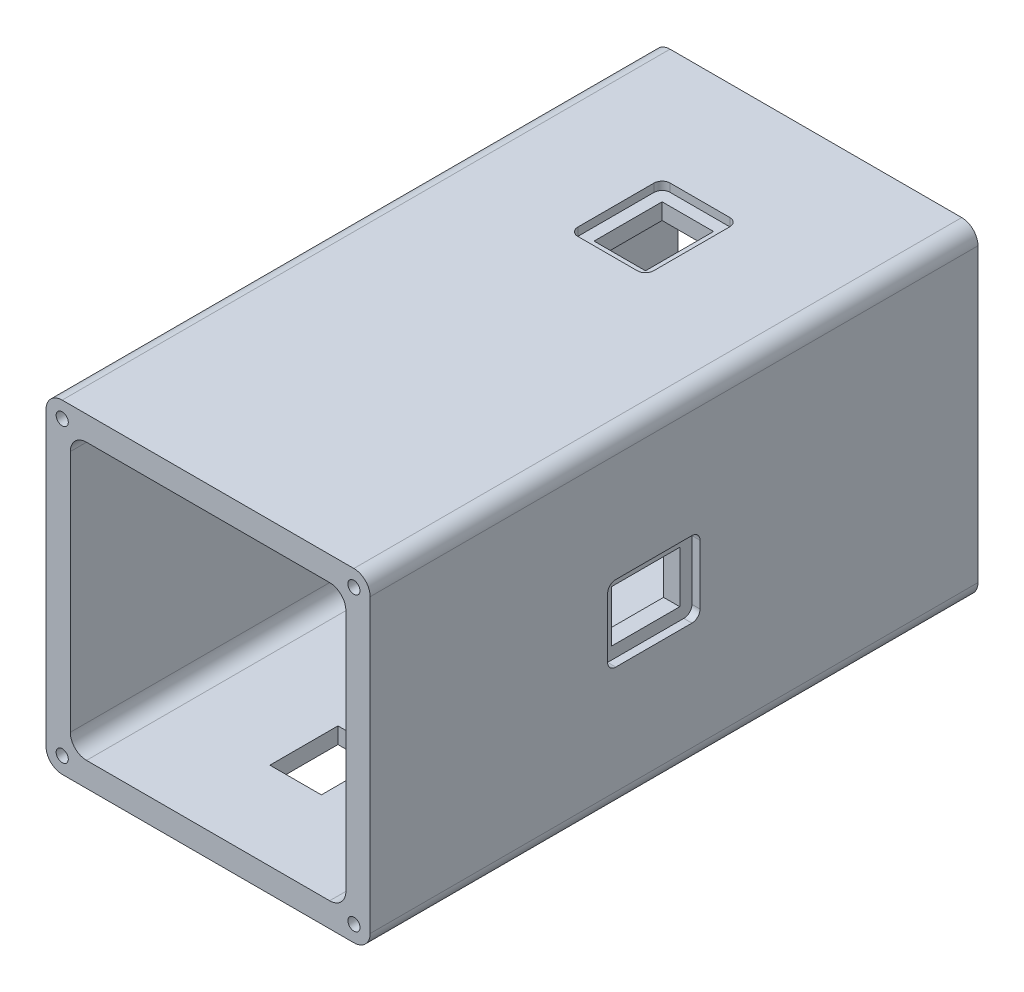
SolidWorks part; units mm, degrees
ref_plane "Front Plane" through (0, 0, 0) normal (0, 0, 1) x (1, 0, 0)
ref_plane "Top Plane" through (0, 0, 0) normal (0, 1, 0) x (1, 0, 0)
ref_plane "Right Plane" through (0, 0, 0) normal (1, 0, 0) x (0, 0, -1)
sketch "Sketch1" plane through (0, 0, 0) normal (0, 0, 1) x (1, 0, 0)
  line L104 (10.5727, 43.58) -> (10.5727, -28.42)
  line L117 (14.5727, -32.42) -> (86.5726, -32.42)
  line L130 (90.5727, -28.4199) -> (90.5727, 43.5589)
  line L143 (86.5517, 47.58) -> (14.5726, 47.58)
  line L212 (16.5727, 37.58) -> (16.5727, -22.42)
  line L213 (20.5727, -26.42) -> (80.5726, -26.42)
  line L214 (84.5726, -22.42) -> (84.5726, 37.58)
  line L215 (80.5726, 41.58) -> (20.5727, 41.58)
  arc A0 (90.5727, 43.5589) -> (86.5517, 47.58) centre (86.5517, 43.5589) ccw
  arc A1 (10.5727, -28.42) -> (14.5727, -32.42) centre (14.5727, -28.42) ccw
  arc A2 (10.5727, 43.58) -> (14.5726, 47.58) centre (14.5726, 43.58) cw
  arc A3 (86.5726, -32.42) -> (90.5727, -28.4199) centre (86.5726, -28.4199) ccw
  arc A4 (80.5726, -26.42) -> (84.5726, -22.42) centre (80.5726, -22.42) ccw
  arc A5 (84.5726, 37.58) -> (80.5726, 41.58) centre (80.5726, 37.58) ccw
  arc A6 (16.5727, 37.58) -> (20.5727, 41.58) centre (20.5727, 37.58) cw
  arc A7 (16.5727, -22.42) -> (20.5727, -26.42) centre (20.5727, -22.42) ccw
  dimension "D1" = 4
extrude "Boss-Extrude1" add sketch "Sketch1" along normal up to surface (150 mm away)
sketch "Sketch2" plane through (0, 0, 150) normal (0, 0, 1) x (1, 0, 0)
  circle A0 centre (14.5727, -28.42) radius 1.5
  circle A1 centre (14.5726, 43.58) radius 1.5
  circle A2 centre (86.5517, 43.5589) radius 1.5003
  circle A3 centre (86.5726, -28.4199) radius 1.5
extrude "Cut-Extrude1" cut sketch "Sketch2" against normal blind 5
ref_plane "Plane1" through (0, 0, 75) normal (0, 0, -1) x (-1, 0, 0)
mirror "Mirror1" about plane through (0, 0, 75) normal (0, 0, -1) of "Cut-Extrude1"
ref_plane "Plane3" through (50.5727, 0, 0) normal (-1, 0, 0) x (0, 0, 1)
sketch "Sketch7" plane through (0, 47.58, 0) normal (0, 1, 0) x (1, 0, 0)
  line L0 (50.5622, -31.6) -> (50.5622, 0) construction
  line L1 (56.9122, -48.4) -> (44.2122, -48.4)
  line L2 (56.9122, -48.4) -> (56.9122, -31.6)
  line L3 (56.9122, -31.6) -> (44.2122, -31.6)
  line L4 (44.2122, -48.4) -> (44.2122, -31.6)
  line L5 (86.5517, 0) -> (14.5726, 0) construction
  line L6 (56.9122, -40) -> (44.2122, -40) construction
  dimension "D1" = 16.8
  dimension "D2" = 12.7
  dimension "D3" = 40
extrude "Cut-Extrude2" cut sketch "Sketch7" against normal blind 13
sketch "Sketch8" plane through (90.5727, 0, 0) normal (1, 0, 0) x (0, 0, -1)
  line L0 (-71.6, 7.5695) -> (-150, 7.5695) construction
  line L1 (-71.6, 13.9195) -> (-71.6, 1.2195)
  line L2 (-71.6, 13.9195) -> (-88.4, 13.9195)
  line L3 (-88.4, 13.9195) -> (-88.4, 1.2195)
  line L4 (-71.6, 1.2195) -> (-88.4, 1.2195)
  line L5 (-80, 13.9195) -> (-80, 1.2195) construction
  line L6 (-150, -28.4199) -> (-150, 43.5589) construction
  line L7 (0, -28.4199) -> (0, 43.5589) construction
  dimension "D1" = 16.8
  dimension "D2" = 12.7
  dimension "D3" = 78.4
  dimension "D4" = 80
extrude "Cut-Extrude3" cut sketch "Sketch8" against normal blind 13
sketch "Sketch9" plane through (0, -32.42, 0) normal (0, -1, 0) x (1, 0, 0)
  line L0 (50.5726, 128.4) -> (50.5726, 150) construction
  line L1 (56.9226, 111.6) -> (44.2226, 111.6)
  line L2 (56.9226, 111.6) -> (56.9226, 128.4)
  line L3 (56.9226, 128.4) -> (44.2226, 128.4)
  line L4 (44.2226, 111.6) -> (44.2226, 128.4)
  line L5 (56.9226, 120) -> (44.2226, 120) construction
  line L6 (14.5727, 150) -> (86.5726, 150) construction
  line L7 (14.5727, 0) -> (86.5726, 0) construction
  dimension "D1" = 16.8
  dimension "D2" = 12.7
  dimension "D3" = 120
extrude "Cut-Extrude4" cut sketch "Sketch9" against normal blind 13
sketch "Sketch10" plane through (0, 47.58, 0) normal (0, 1, 0) x (1, 0, 0)
  line L9 (59.9122, -28.6) -> (41.2122, -28.6)
  line L10 (41.2122, -28.6) -> (41.2122, -51.4)
  line L11 (41.2122, -51.4) -> (59.9122, -51.4)
  line L12 (59.9122, -51.4) -> (59.9122, -28.6)
  line L13 (59.9122, -28.6) -> (41.2122, -28.6)
  line L14 (41.2122, -28.6) -> (41.2122, -51.4)
  line L15 (41.2122, -51.4) -> (59.9122, -51.4)
  line L16 (59.9122, -51.4) -> (59.9122, -28.6)
  dimension "D1" = 3
extrude "Cut-Extrude5" cut sketch "Sketch10" against normal blind 2
fillet "Fillet1" radius 2 4 edges at (41.2122, 46.58, 51.4) (41.2122, 46.58, 28.6) (59.9122, 46.58, 28.6) (59.9122, 46.58, 51.4)
sketch "Sketch12" plane through (90.5727, 0, 0) normal (1, 0, 0) x (0, 0, -1)
  line L8 (-91.4, 16.9195) -> (-91.4, -1.7805)
  line L9 (-91.4, -1.7805) -> (-68.6, -1.7805)
  line L10 (-68.6, 16.9195) -> (-91.4, 16.9195)
  line L11 (-68.6, -1.7805) -> (-68.6, 16.9195)
  line L12 (-91.4, 16.9195) -> (-91.4, -1.7805)
  line L13 (-91.4, -1.7805) -> (-68.6, -1.7805)
  line L14 (-68.6, 16.9195) -> (-91.4, 16.9195)
  line L15 (-68.6, -1.7805) -> (-68.6, 16.9195)
  dimension "D1" = 3
extrude "Cut-Extrude6" cut sketch "Sketch12" against normal blind 2
fillet "Fillet2" radius 2 4 edges at (89.5727, 16.9195, 68.6) (89.5727, -1.7805, 68.6) (89.5727, 16.9195, 91.4) (89.5727, -1.7805, 91.4)
sketch "Sketch13" plane through (0, -32.42, 0) normal (0, -1, 0) x (1, 0, 0)
  line L8 (41.2226, 108.6) -> (59.9226, 108.6)
  line L9 (41.2226, 131.4) -> (41.2226, 108.6)
  line L10 (59.9226, 108.6) -> (59.9226, 131.4)
  line L11 (59.9226, 131.4) -> (41.2226, 131.4)
  line L12 (41.2226, 108.6) -> (59.9226, 108.6)
  line L13 (41.2226, 131.4) -> (41.2226, 108.6)
  line L14 (59.9226, 108.6) -> (59.9226, 131.4)
  line L15 (59.9226, 131.4) -> (41.2226, 131.4)
  dimension "D1" = 3
extrude "Cut-Extrude7" cut sketch "Sketch13" against normal blind 2
fillet "Fillet3" radius 2 4 edges at (41.2226, -31.42, 108.6) (59.9226, -31.42, 108.6) (59.9226, -31.42, 131.4) (41.2226, -31.42, 131.4)
